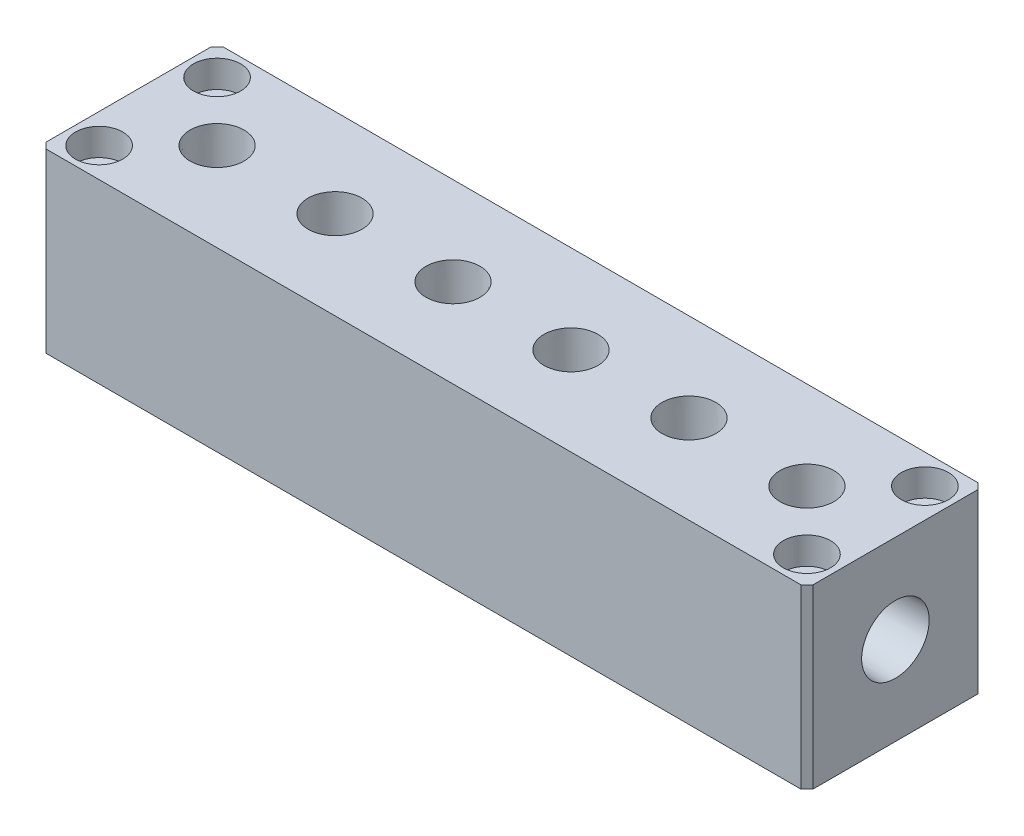
from build123d import *

# Parameters (mm, degrees)
SKETCH_1_W                = 130
SKETCH_1_H                = 30
EXTRUDE_1_DEPTH           = 15
F_1_8_RC_1_AT_2_COUNT     = 2
F_1_8_RC_1_AT_2_PITCH     = 20
F_1_8_RC_1_AT_3_COUNT     = 2
F_1_8_RC_1_AT_3_PITCH     = 40
F_1_8_RC_1_AT_4_COUNT     = 2
F_1_8_RC_1_AT_4_PITCH     = 60
F_1_8_RC_1_AT_5_COUNT     = 2
F_1_8_RC_1_AT_5_PITCH     = 80
F_1_8_RC_1_AT_6_COUNT     = 2
F_1_8_RC_1_AT_6_PITCH     = 100
CHAMFER_1_SIZE            = 1
HOLE_WIZARD_1_D           = 4.5
HOLE_WIZARD_1_CBORE_D     = 8
HOLE_WIZARD_1_CBORE_DEPTH = 4.6


with BuildPart() as part:
    # 草图1 → 凸台-拉伸1 (new, symmetric)
    with BuildSketch(Plane(origin=(0, 0, 0), x_dir=(1, 0, 0), z_dir=(0, 1, 0))):
        Rectangle(SKETCH_1_W, SKETCH_1_H)
    extrude(amount=EXTRUDE_1_DEPTH, both=True)

    # 草图4 → 1/4 Rc 螺纹孔1 (revolve, cut)
    with BuildSketch(Plane(origin=(65, 0, 0), x_dir=(0, 0, -1), z_dir=(0, 1, 0))):
        Polygon((0, 0), (0, 123.214604312), (5.35, 120), (5.35, 11), (5.379117168, 11), (5.7225, 0), align=None)
    revolve(axis=Axis((71.35, 0, 0), (-1, 0, 0)), mode=Mode.SUBTRACT)

    # 草图8 → 1/8 Rc 螺纹孔1 (revolve, cut)
    with BuildSketch(Plane(origin=(50, 15, 0), x_dir=(0, 0, 1), z_dir=(1, 0, 0))):
        Polygon((0, 0), (0, 14.313399445), (3.95, 11.94), (3.95, 7.4), (4.342497004, 7.4), (4.5735, 0), align=None)
    f_1_8_rc_1 = revolve(axis=Axis((50, 21.35, 0), (0, -1, 0)), mode=Mode.SUBTRACT)

    # 1/8 Rc 螺纹孔1 at 2: 1/8 Rc 螺纹孔1 ×2
    with Locations(*[(-i * F_1_8_RC_1_AT_2_PITCH, 0, 0) for i in range(1, F_1_8_RC_1_AT_2_COUNT)]):
        add(f_1_8_rc_1, mode=Mode.SUBTRACT)

    # 1/8 Rc 螺纹孔1 at 3: 1/8 Rc 螺纹孔1 ×2
    with Locations(*[(-i * F_1_8_RC_1_AT_3_PITCH, 0, 0) for i in range(1, F_1_8_RC_1_AT_3_COUNT)]):
        add(f_1_8_rc_1, mode=Mode.SUBTRACT)

    # 1/8 Rc 螺纹孔1 at 4: 1/8 Rc 螺纹孔1 ×2
    with Locations(*[(-i * F_1_8_RC_1_AT_4_PITCH, 0, 0) for i in range(1, F_1_8_RC_1_AT_4_COUNT)]):
        add(f_1_8_rc_1, mode=Mode.SUBTRACT)

    # 1/8 Rc 螺纹孔1 at 5: 1/8 Rc 螺纹孔1 ×2
    with Locations(*[(-i * F_1_8_RC_1_AT_5_PITCH, 0, 0) for i in range(1, F_1_8_RC_1_AT_5_COUNT)]):
        add(f_1_8_rc_1, mode=Mode.SUBTRACT)

    # 1/8 Rc 螺纹孔1 at 6: 1/8 Rc 螺纹孔1 ×2
    with Locations(*[(-i * F_1_8_RC_1_AT_6_PITCH, 0, 0) for i in range(1, F_1_8_RC_1_AT_6_COUNT)]):
        add(f_1_8_rc_1, mode=Mode.SUBTRACT)

    # 倒角1
    chamfer_1_edges = [part.edges().sort_by_distance(p)[0] for p in [
        (65, 0, 15),
        (-65, 0, 15),
        (-65, 0, -15),
        (65, 0, -15),
    ]]
    chamfer(chamfer_1_edges, length=CHAMFER_1_SIZE)

    # 打孔尺寸(%根据)内六角圆柱头螺钉的类型1 (through all)
    with Locations(Plane(origin=(0, 15, 0), x_dir=(1, 0, 0), z_dir=(0, 1, 0))):
        with Locations((-60, 10), (-60, -10), (60, -10), (60, 10)):
            CounterBoreHole(HOLE_WIZARD_1_D / 2, HOLE_WIZARD_1_CBORE_D / 2, HOLE_WIZARD_1_CBORE_DEPTH)


solid = part.part
